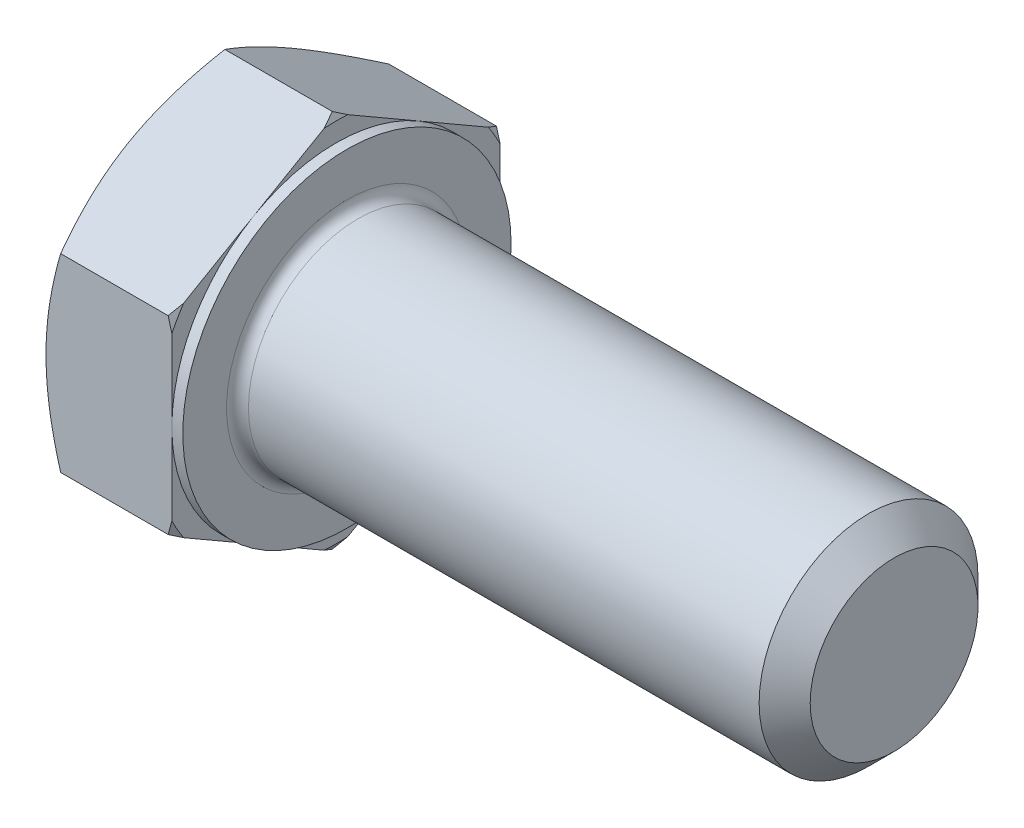
from build123d import *

# Parameters (mm, degrees)
EXTRUDE_368_DEPTH = 7.5
SKETCH_4_W        = 0.6
SKETCH_4_H        = 11.392304845
CHAMFER_1891_SIZE = 1.4
FILLET_1936_R     = 0.6


with BuildPart() as part:
    # 草图1 → Extrude 368 (new body)
    with BuildSketch(Plane(origin=(0, 0, 0), x_dir=(0, 0, -1), z_dir=(1, 0, 0))):
        Polygon((9, 5.196152423), (9, -5.196152423), (0, -10.392304845), (-9, -5.196152423), (-9, 5.196152423), (0, 10.392304845), align=None)
    extrude(amount=EXTRUDE_368_DEPTH)

    # 草图2 → 凸台-旋转1 (revolve)
    with BuildSketch(Plane.XY, mode=Mode.PRIVATE) as revolve_1_sk:
        Polygon((0, 0), (37.5, 0), (37.5, 4.4845), (37.5, 6), (0, 6), align=None)
    revolve(revolve_1_sk.sketch.rotate(Axis((0, 0, 0), (1, 0, 0)), 90), axis=Axis((0, 0, 0), (1, 0, 0)))

    # 草图3 → 切除-旋转1 (revolve, cut)
    with BuildSketch(Plane.XY):
        Polygon((0, 9), (3.690598923, 15.392304845), (3.690598923, 20.392304845), (-10, 20.392304845), (-10, 9), align=None)
    revolve(axis=Axis((0, 0, 0), (1, 0, 0)), mode=Mode.SUBTRACT)

    # 草图5 → 切除-旋转2 (revolve, cut)
    with BuildSketch(Plane.XY):
        Polygon((7.5, 9), (3.809401077, 15.392304845), (3.809401077, 20.392304845), (13.809401077, 20.392304845), (13.809401077, 9), align=None)
    revolve(axis=Axis((0, 0, 0), (1, 0, 0)), mode=Mode.SUBTRACT)

    # 草图4 → 切除-旋转3 (revolve, cut)
    with BuildSketch(Plane.XY, mode=Mode.PRIVATE) as cut_revolve_3_sk:
        with Locations((7.2, 14.696152423)):
            Rectangle(SKETCH_4_W, SKETCH_4_H)
    revolve(cut_revolve_3_sk.sketch.rotate(Axis((0, 0, 0), (1, 0, 0)), 270), axis=Axis((0, 0, 0), (1, 0, 0)), mode=Mode.SUBTRACT)

    # Chamfer 1891
    chamfer_1891_edges = [part.edges().sort_by_distance(p)[0] for p in [
        (37.5, 0, -6),
    ]]
    chamfer(chamfer_1891_edges, length=CHAMFER_1891_SIZE)

    # Fillet 1936
    fillet_1936_edges = [part.edges().sort_by_distance(p)[0] for p in [
        (7.5, 0, -6),
    ]]
    fillet(fillet_1936_edges, radius=FILLET_1936_R)


solid = part.part
